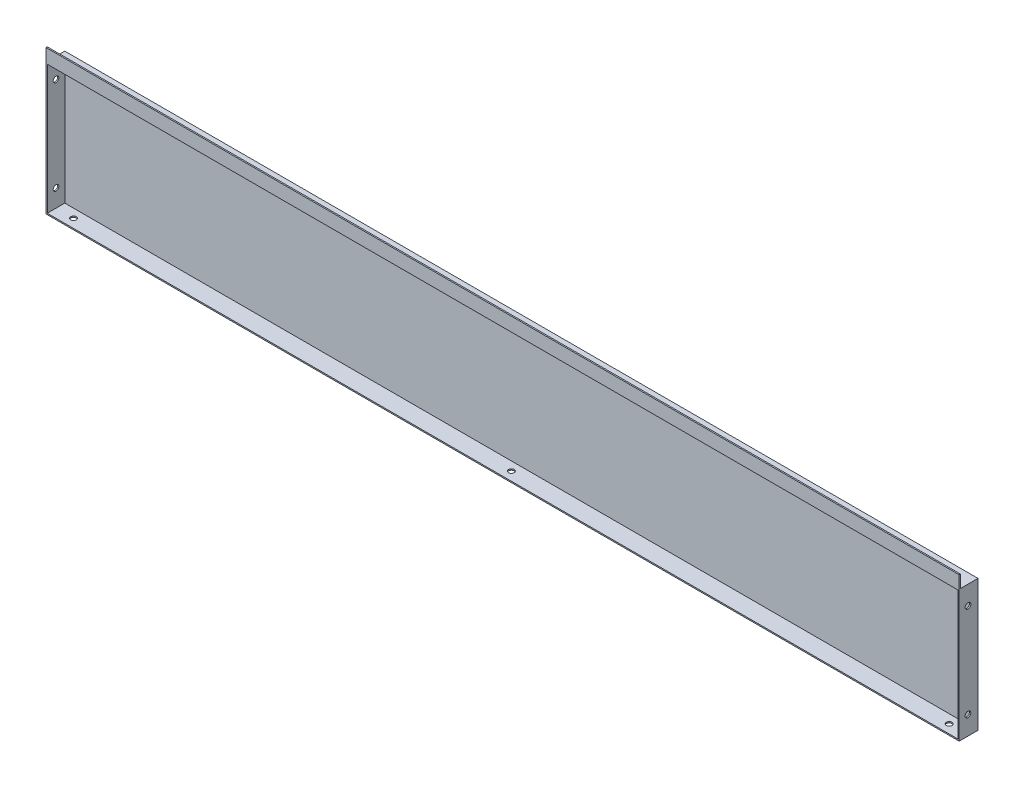
SolidWorks part; units mm, degrees
ref_plane "前视基准面" through (0, 0, 0) normal (0, 0, 1) x (1, 0, 0)
ref_plane "上视基准面" through (0, 0, 0) normal (0, 1, 0) x (1, 0, 0)
ref_plane "右视基准面" through (0, 0, 0) normal (1, 0, 0) x (0, 0, -1)
sketch "草图1" plane through (0, 0, 0) normal (0, 0, 1) x (1, 0, 0)
  line L1 (0, 0) -> (1457, 0)
  line L2 (0, 0) -> (0, 210)
  line L3 (0, 210) -> (1457, 210)
  line L4 (1457, 0) -> (1457, 210)
  dimension "D1" = 210
  dimension "D2" = 1457
extrude "凸台-拉伸1" add sketch "草图1" along normal blind 30
shell "抽壳1" thickness 2
sketch "草图2" plane through (0, 0, 30) normal (0, 0, 1) x (1, 0, 0)
  line L0 (1455, 208) -> (2, 208) construction
  line L1 (0, 230) -> (1457, 230)
  line L2 (0, 230) -> (0, 210)
  line L3 (0, 210) -> (1457, 210)
  line L4 (1457, 210) -> (1457, 230)
  line L6 (1457, 210) -> (0, 210) construction
  dimension "D1" = 20
extrude "凸台-拉伸2" add sketch "草图2" against normal blind 2
sketch "草图3" plane through (0, 2, 0) normal (0, 1, 0) x (1, 0, 0)
  line L0 (2, -16) -> (1533.8827, -16) construction
  line L1 (2, -30) -> (2, -2) construction
  line L2 (728.5, -30) -> (728.5, 440.2854) construction
  line L3 (2, -30) -> (1455, -30) construction
  line L4 (0, -30) -> (0, 0) construction
  line L5 (1457, -30) -> (1457, 0) construction
  circle A0 centre (1427, -16) radius 4.5
  circle A1 centre (728.5, -16) radius 4.5
  circle A2 centre (30, -16) radius 4.5
  dimension "D1" = 9
  dimension "D2" = 30
  dimension "D3" = 9
  dimension "D4" = 30
  dimension "D5" = 9
extrude "切除-拉伸1" cut sketch "草图3" against normal blind 10
sketch "草图4" plane through (2, 0, 0) normal (1, 0, 0) x (0, 0, -1)
  line L0 (-16, 2) -> (-16, 242.3088) construction
  line L1 (-30, 2) -> (-2, 2) construction
  line L2 (-30, 0) -> (0, 0) construction
  line L3 (-28, 210) -> (0, 210) construction
  circle A0 centre (-16, 30) radius 4.5
  circle A1 centre (-16, 180) radius 4.5
  dimension "D1" = 9
  dimension "D2" = 9
  dimension "D3" = 30
  dimension "D4" = 30
extrude "切除-拉伸2" cut sketch "草图4" against normal blind 76 and the other way blind 1525
